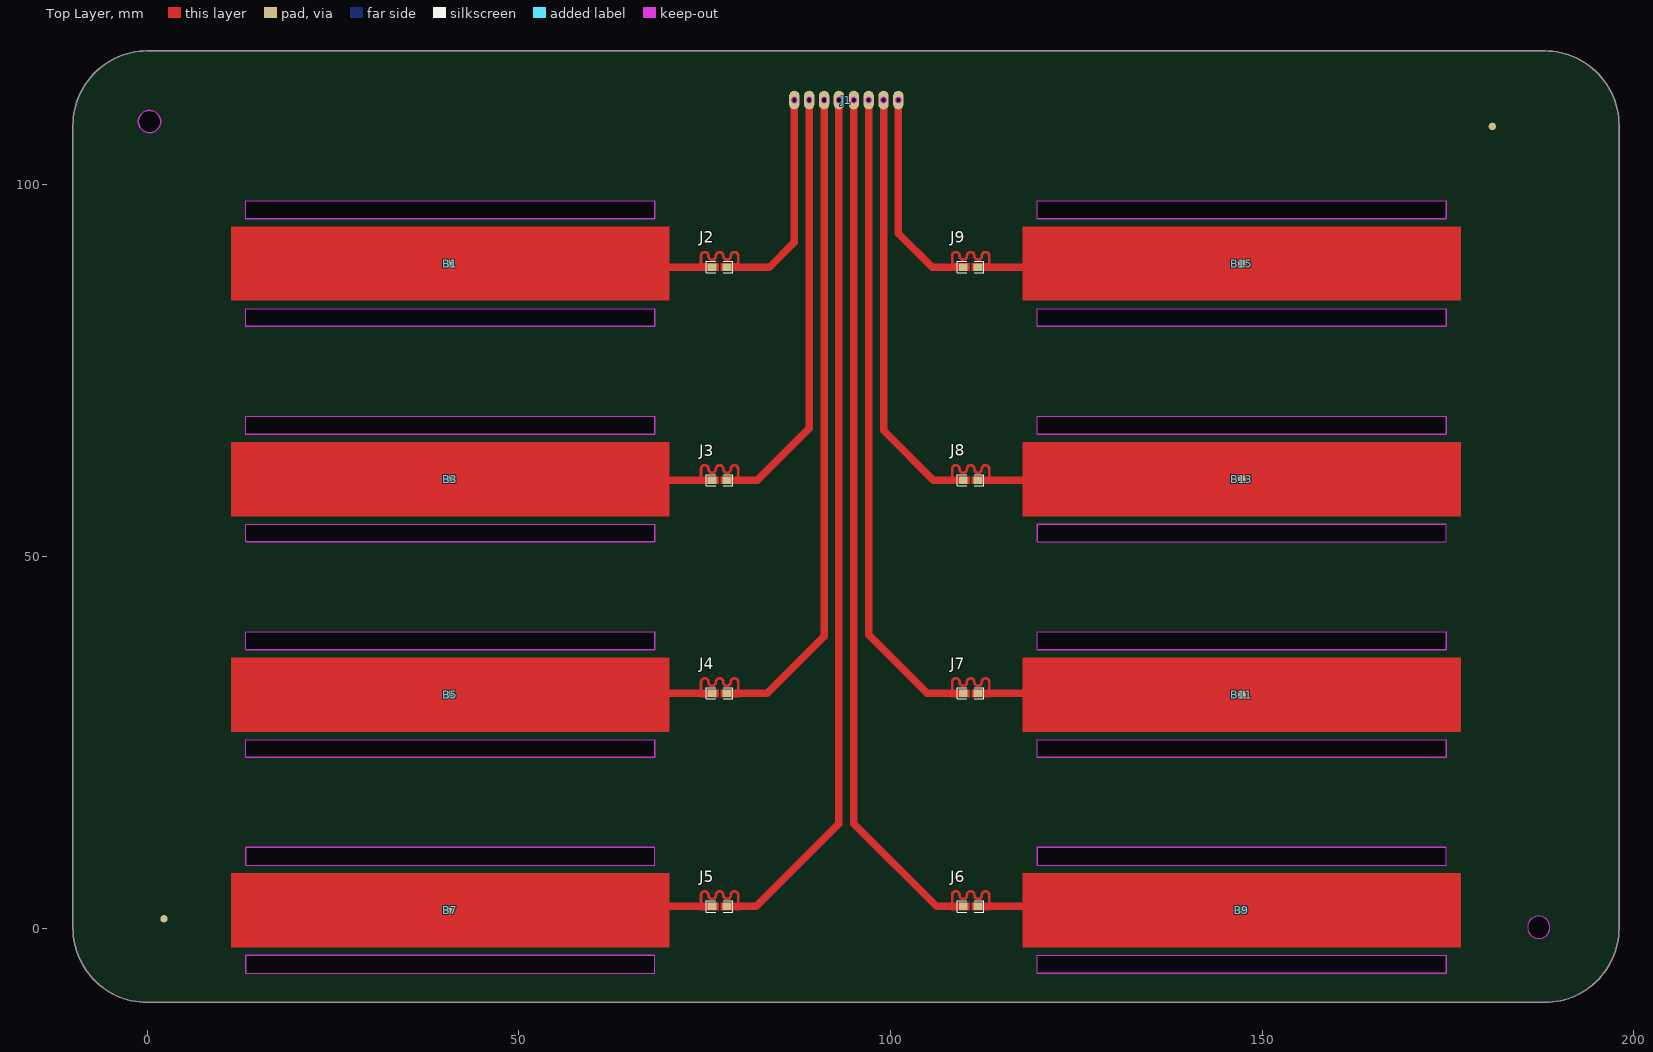
[diagram p0: Top Layer view]
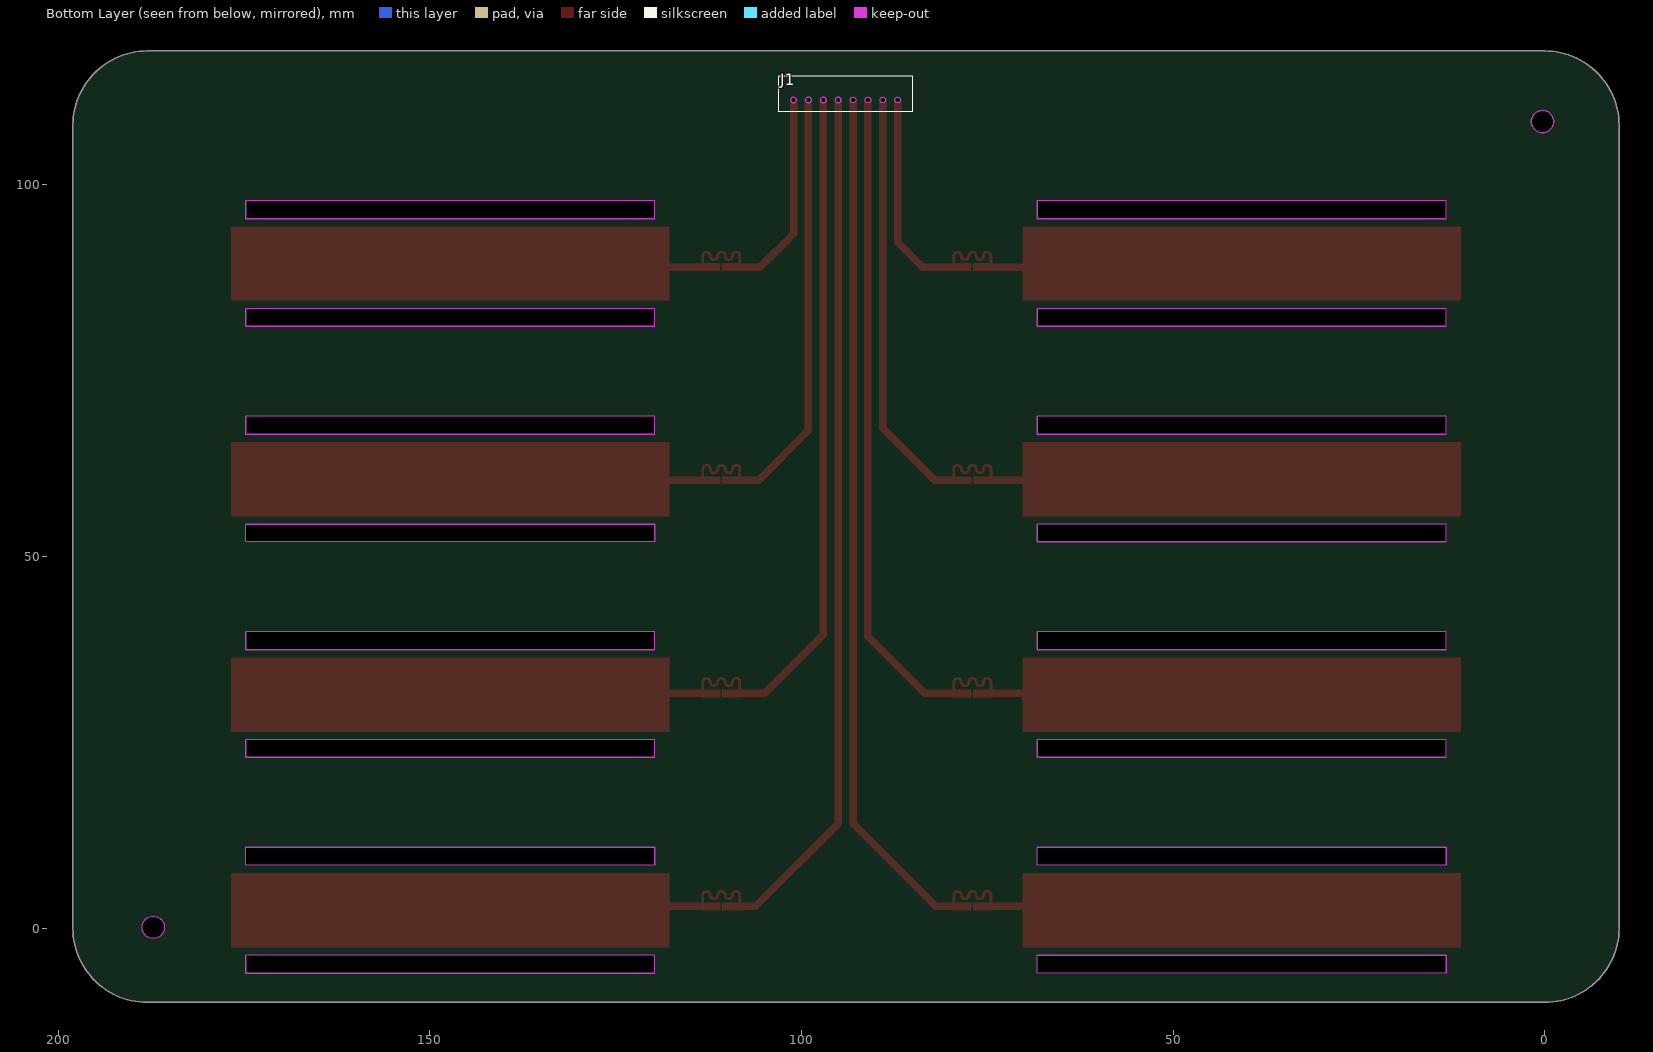
[diagram p1: Bottom Layer view, seen from below]
# Altium PCB MISC86336.PcbDoc
Units mm, origin at the board's own origin, x right, y up, seen from the top; angles counter-clockwise.
Board outline 208 x 128 mm, 2 copper layers (Top Layer, Bottom Layer); 17 components, 8 nets, 42 pads, 0 vias.

## Layer stack, top to bottom (the 12.6 mil dielectric is the usual default, probably not edited)
Top Solder: solder mask 0.0102, Solder Resist, Dk 3.5
Top Layer: signal copper 0.0356
Dielectric 1: dielectric 0.32, FR-4, Dk 4.8
Bottom Layer: signal copper 0.0356
Bottom Solder: solder mask 0.0102, Solder Resist, Dk 3.5

## Board outline
-10,0 -10,108 cw(c0,108) 0,118 188,118 cw(c188,108) 198,108 198,0 cw(c188,0) 188,-10 0,-10 cw(c0,0)
cut-out: 185.7,0.1 ccw(c187.2,0.1) 187.2,-1.4 ccw(c187.2,0.1) 188.7,0.1 ccw(c187.2,0.1) 187.2,1.6 ccw(c187.2,0.1)
cut-out: 0.3,107 cw(c0.3,108.5) -1.2,108.5 cw(c0.3,108.5) 0.3,110 cw(c0.3,108.5) 1.8,108.5 cw(c0.3,108.5)
cut-out: 119.75,-6.05 119.75,-3.65 174.75,-3.65 174.75,-6.05
cut-out: 119.75,8.45 174.75,8.45 174.75,10.85 119.75,10.85
cut-out: 119.75,22.95 119.75,25.35 174.75,25.35 174.75,22.95
cut-out: 119.75,37.45 119.75,39.85 174.75,39.85 174.75,37.45
cut-out: 119.75,51.95 174.75,51.95 174.75,54.35 119.75,54.35
cut-out: 119.75,66.45 119.75,68.85 174.75,68.85 174.75,66.45
cut-out: 119.75,80.95 119.75,83.35 174.75,83.35 174.75,80.95
cut-out: 119.75,95.45 119.75,97.85 174.75,97.85 174.75,95.45
cut-out: 13.25,95.45 13.25,97.85 68.25,97.85 68.25,95.45
cut-out: 13.25,80.95 13.25,83.35 68.25,83.35 68.25,80.95
cut-out: 13.25,66.45 13.25,68.85 68.25,68.85 68.25,66.45
cut-out: 13.25,51.95 13.25,54.35 68.25,54.35 68.25,51.95
cut-out: 13.25,37.45 13.25,39.85 68.25,39.85 68.25,37.45
cut-out: 13.25,22.95 13.25,25.35 68.25,25.35 68.25,22.95
cut-out: 13.25,8.45 68.25,8.45 68.25,10.85 13.25,10.85
cut-out: 13.25,-6.05 68.25,-6.05 68.25,-3.65 13.25,-3.65

## Design rules (kind name [scope] priority, off if disabled: settings)
Clearance [All] p1: gap=0.01 ignorepadtopadclearanceinfootprint=FALSE
ComponentClearance [All] p1: gap=0 collisioncheckmode=3 verticalgap=0 showdistances=FALSE
HoleToHoleClearance [All] p1: gap=0 allowstackedmicrovias=TRUE
MinimumSolderMaskSliver [All] p1: minsoldermaskwidth=0
PolygonConnect [All] p1: connectstyle=Direct reliefconductorwidth=0.254 reliefentries=4 polygonreliefangle="90 Angle" airgapwidth=0.254
RoutingVias [All] p1: holewidth=0.711 width=1.27 viastyle="Through Hole" minholewidth=0.711 minwidth=1.27 maxholewidth=0.711 maxwidth=1.27
SilkToSilkClearance [All] p1: silktosilkclearance=0
SilkToSolderMaskClearance [IsPad] p1: minsilkscreentomaskgap=0 clearancetoexposedcopper=TRUE
SolderMaskExpansion [All] p1: expansion=0.102 istentingtop=FALSE
Width [All] p1: maxlimit=2 minlimit=0.254 preferedwidth=0.254 minimp=50.000000 maximp=50.000000 favimp=50.000000
25 further rules are at their usual default settings.

## Components (designator, comment, footprint, x,y, rotation, side; value= is the part's Value field where it differs from the comment)
B1 "Pth" 55*10*1MM 40.75,89.4 r180 top locked
B3 "Pth" 55*10*1MM 40.75,60.4 r180 top locked
B5 "Pth" 55*10*1MM 40.75,31.4 r180 top locked
B7 "Pth" 55*10*1MM 40.75,2.4 r180 top locked
B9 "Pth" 55*10*1MM 147.25,2.4 r180 top locked
B11 "Pth" 55*10*1MM 147.25,31.4 r180 top locked
B13 "Pth" 55*10*1MM 147.25,60.4 r180 top locked
B15 "Pth" 55*10*1MM 147.25,89.4 r180 top locked
J1 "HX-2.0mm-8P THT connector with latch" HX2.0-8P 94.05,111.4 r0 bottom locked
J2 "FPC" 异形电阻 76.996,88.917 r90 top
J3 "FPC" 异形电阻 76.996,60.25 r90 top
J4 "FPC" 异形电阻 76.996,31.584 r90 top
J5 "FPC" 异形电阻 76.996,2.917 r90 top
J6 "FPC" 异形电阻 110.771,2.917 r90 top
J7 "FPC" 异形电阻 110.771,31.584 r90 top
J8 "FPC" 异形电阻 110.771,60.25 r90 top
J9 "FPC" 异形电阻 110.771,88.917 r90 top

## Footprints (in the part's own frame and the unit in brackets; to place one, negate y for a bottom-side part, rotate by r counter-clockwise, add the part's x,y. Pads: shape width x height; smd on the part's side, far side on the other; paste and mask are expansions set on the pad)
55*10*1MM [mm]
  rect 1x1 smd: 1(0,0)
  Top Layer region: -29.499,-5 29.501,-5 29.501,5 -29.499,5
HX2.0-8P [mm]
  oval 1.4x2.5 smd far side: 1(-7,0) 2(-5,0) 3(-3,0) 4(-1,0) 5(1,0) 6(3,0) 7(5,0) 8(7,0)
  round 0.75 hole 0.75: 1(-7,0) 2(-5,0) 3(-3,0) 4(-1,0) 5(1,0) 6(3,0) 7(5,0) 8(7,0)
  Keep-Out Layer board cut-out: -7,-0.375 -7.144,-0.346 -7.265,-0.265 -7.346,-0.144 -7.375,0 -7.375,0 -7.346,0.144 -7.265,0.265 -7.144,0.346 -7,0.375 -7,0.375 -6.856,0.346 -6.735,0.265 -6.654,0.144 -6.625,0 -6.625,0 -6.654,-0.144 -6.735,-0.265 -6.856,-0.346 -7,-0.375
  Keep-Out Layer board cut-out: -3,-0.375 -3.144,-0.346 -3.265,-0.265 -3.346,-0.144 -3.375,0 -3.375,0 -3.346,0.144 -3.265,0.265 -3.144,0.346 -3,0.375 -3,0.375 -2.856,0.346 -2.735,0.265 -2.654,0.144 -2.625,0 -2.625,0 -2.654,-0.144 -2.735,-0.265 -2.856,-0.346 -3,-0.375
  Keep-Out Layer board cut-out: -1,-0.375 -1.144,-0.346 -1.265,-0.265 -1.346,-0.144 -1.375,0 -1.375,0 -1.346,0.144 -1.265,0.265 -1.144,0.346 -1,0.375 -1,0.375 -0.856,0.346 -0.735,0.265 -0.654,0.144 -0.625,0 -0.625,0 -0.654,-0.144 -0.735,-0.265 -0.856,-0.346 -1,-0.375
  Keep-Out Layer board cut-out: 0.625,0 0.654,-0.144 0.735,-0.265 0.856,-0.346 1,-0.375 1,-0.375 1.144,-0.346 1.265,-0.265 1.346,-0.144 1.375,0 1.375,0 1.346,0.144 1.265,0.265 1.144,0.346 1,0.375 1,0.375 0.856,0.346 0.735,0.265 0.654,0.144 0.625,0
  Keep-Out Layer board cut-out: 2.625,0 2.654,-0.144 2.735,-0.265 2.856,-0.346 3,-0.375 3,-0.375 3.144,-0.346 3.265,-0.265 3.346,-0.144 3.375,0 3.375,0 3.346,0.144 3.265,0.265 3.144,0.346 3,0.375 3,0.375 2.856,0.346 2.735,0.265 2.654,0.144 2.625,0
  Keep-Out Layer board cut-out: 4.625,0 4.654,-0.144 4.735,-0.265 4.856,-0.346 5,-0.375 5,-0.375 5.144,-0.346 5.265,-0.265 5.346,-0.144 5.375,0 5.375,0 5.346,0.144 5.265,0.265 5.144,0.346 5,0.375 5,0.375 4.856,0.346 4.735,0.265 4.654,0.144 4.625,0
  Keep-Out Layer board cut-out: 6.625,0 6.654,-0.144 6.735,-0.265 6.856,-0.346 7,-0.375 7,-0.375 7.144,-0.346 7.265,-0.265 7.346,-0.144 7.375,0 7.375,0 7.346,0.144 7.265,0.265 7.144,0.346 7,0.375 7,0.375 6.856,0.346 6.735,0.265 6.654,0.144 6.625,0
  Keep-Out Layer pour cut-out: -5,-0.375 -5.144,-0.346 -5.265,-0.265 -5.346,-0.144 -5.375,0 -5.375,0 -5.346,0.144 -5.265,0.265 -5.144,0.346 -5,0.375 -5,0.375 -4.856,0.346 -4.735,0.265 -4.654,0.144 -4.625,0 -4.625,0 -4.654,-0.144 -4.735,-0.265 -4.856,-0.346 -5,-0.375
  Keep-Out Layer circle w0.01: c-7,0 r0.375
  Keep-Out Layer circle w0.01: c-5,0 r0.375
  Keep-Out Layer circle w0.01: c-3,0 r0.375
  Keep-Out Layer circle w0.01: c-1,0 r0.375
  Keep-Out Layer circle w0.01: c7,0 r0.375
  Keep-Out Layer circle w0.01: c5,0 r0.375
  Keep-Out Layer circle w0.01: c3,0 r0.375
  Keep-Out Layer circle w0.01: c1,0 r0.375
  silkscreen extent -9,-3.2 9,1.6
异形电阻 [mm]
  rect 1x1.2 smd mask+0: 1(0,1) 2(0,-1)
  Top Layer region: 0.5,0.125 0.5,2.55 0.5,2.575 0.481,2.621 0.446,2.656 0.4,2.675 0.375,2.675 0.375,2.675 -0.425,2.675 -0.44,2.675 -0.467,2.664 -0.489,2.642 -0.5,2.615 -0.5,2.6 -0.5,2.6 -0.5,0.125
  Top Layer region: -0.5,-2.625 -0.5,-2.635 -0.492,-2.653 -0.478,-2.667 -0.46,-2.675 -0.45,-2.675 -0.45,-2.675 0.4,-2.675 0.42,-2.675 0.457,-2.66 0.485,-2.632 0.5,-2.595 0.5,-2.575 0.5,-2.575 0.5,-0.125 -0.5,-0.125 -0.5,-0.125
  Top Layer pour cut-out: -1,3 2.5,3 2.5,-3 -1,-3
  Top Layer lines w0.2: -0.325,2.5 0,2.5
  Top Layer lines w0.35: -0.325,2.5 0,2.5 1.525,2.5 cw(c1.525,2) 1.525,1.5 ; 1.5,1.5 ccw(c1.5,1) 1.5,0.5 ; 1.525,0.5 cw(c1.525,0) 1.525,-0.5 ; 1.5,-0.5 ccw(c1.5,-1) 1.5,-1.5 ; 1.525,-1.5 cw(c1.525,-2) 1.525,-2.5 0,-2.5 -0.325,-2.5
  silkscreen extent -0.98,-2.04 0.95,2.03

## Part data
B1 B3 B5 B7 B9 B11 B13 B15: "Through-hole pad"
J1: library part HX-2.0mm-8P直插带扣

## Free pads (board coordinates)
  round 1 smd: 3(2.246,1.25) 3(180.946,107.85)

## Nets (pads, with @x,y where several pads share a name; then routed paths per layer and width w, separated by ;. In a path a pad name is that pad's centre, name@x,y a point inside that pad or via, vN(x,y) a via of type N, cw(c..) or ccw(c..) an arc to the next point about the centre after c; other vN are vias at no path point)
B1: B1.1 J1.1 J2.1 J2.2 | length 64.3
  Top Layer w1: B1.1@41.233,88.917 74.496,88.917 J2.1 ; J2.2 79.496,88.917 83.712,88.917 87.05,92.255 J1.1@87.05,111.4
B3: B3.1 J1.2 J3.1 J3.2 | length 77.6
  Top Layer w1: 57.5,60.9 58.15,60.25 74.496,60.25 ; 75.218,60.25 74.496,60.25 ; J3.1 74.496,60.25 ; J3.2 79.496,60.25 82.046,60.25 89.05,67.255 J1.2@89.05,111.4
B5: B5.1 J1.3 J4.1 J4.2 | length 123.7
  Top Layer w1: B5.1 40.934,31.584 74.496,31.584 J4.1 ; J4.2 79.496,31.584 83.379,31.584 91.05,39.255 J1.3@91.05,111.4
B7: B7.1 J1.4 J5.1 J5.2 | length 152.5
  Top Layer w1: B7.1 41.267,2.917 74.496,2.917 J5.1 ; J5.2 79.496,2.917 81.912,2.917 93.05,14.055 J1.4@93.05,111.4
B9: B9.1 J1.5 J6.1 J6.2 | length 152.4
  Top Layer w1: J1.5@95.05,111.4 95.05,14.046 106.179,2.917 108.271,2.917 J6.1 ; J6.2 113.271,2.917 120.829,2.917 121.346,2.4 B9.1
B11: B11.1 J1.6 J7.1 J7.2 | length 123.5
  Top Layer w1: J1.6@97.05,111.4 97.05,39.446 104.912,31.584 108.271,31.584 J7.1 ; J7.2 113.271,31.584 147.066,31.584 B11.1
B13: B13.1 J1.7 J8.1 J8.2 | length 93.5
  Top Layer w1: J1.7@99.05,111.4 99.05,66.946 105.746,60.25 108.271,60.25 J8.1 ; J8.2 113.271,60.25 147.1,60.25 B13.1
B15: B15.1 J1.8 J9.1 J9.2 | length 64.2
  Top Layer w1: J1.8@101.05,111.4 101.05,93.446 105.579,88.917 108.271,88.917 J9.1 ; J9.2 113.271,88.917 146.767,88.917 B15.1

## Keep-outs
Keep-Out Layer:
  circle w0.1: c0.3,108.5 r1.5
  circle w0.1: c187.2,0.1 r1.5
  lines w0.013: -10,0 ccw(c0,0) 0,-10 188,-10 ccw(c188,0) 198,0 198,108 ccw(c188,108) 188,118 0,118 ccw(c0,108) -10,108 -10,0 ; 13.25,-6.05 13.25,-3.65 68.25,-3.65 68.25,-6.05 13.25,-6.05 ; 13.25,8.45 13.25,10.85 68.25,10.85 68.25,8.45 13.25,8.45 ; 13.25,22.95 13.25,25.35 68.25,25.35 68.25,22.95 13.25,22.95 ; 13.25,37.45 13.25,39.85 68.25,39.85 68.25,37.45 13.25,37.45 ; 13.25,51.95 13.25,54.35 68.25,54.35 68.25,51.95 13.25,51.95 ; 13.25,66.45 13.25,68.85 68.25,68.85 68.25,66.45 13.25,66.45 ; 13.25,80.95 13.25,83.35 68.25,83.35 68.25,80.95 13.25,80.95 ; 13.25,95.45 13.25,97.85 68.25,97.85 68.25,95.45 13.25,95.45 ; 119.75,-6.05 174.75,-6.05 174.75,-3.65 119.75,-3.65 119.75,-6.05 ; 119.75,8.45 174.75,8.45 174.75,10.85 119.75,10.85 119.75,8.45 ; 119.75,22.95 174.75,22.95 174.75,25.35 119.75,25.35 119.75,22.95 ; 119.75,37.45 174.75,37.45 174.75,39.85 119.75,39.85 119.75,37.45 ; 119.75,51.95 174.75,51.95 174.75,54.35 119.75,54.35 119.75,51.95 ; 119.75,66.45 174.75,66.45 174.75,68.85 119.75,68.85 119.75,66.45 ; 119.75,80.95 119.75,83.35 174.75,83.35 174.75,80.95 119.75,80.95 ; 119.75,95.45 119.75,97.85 174.75,97.85 174.75,95.45 119.75,95.45